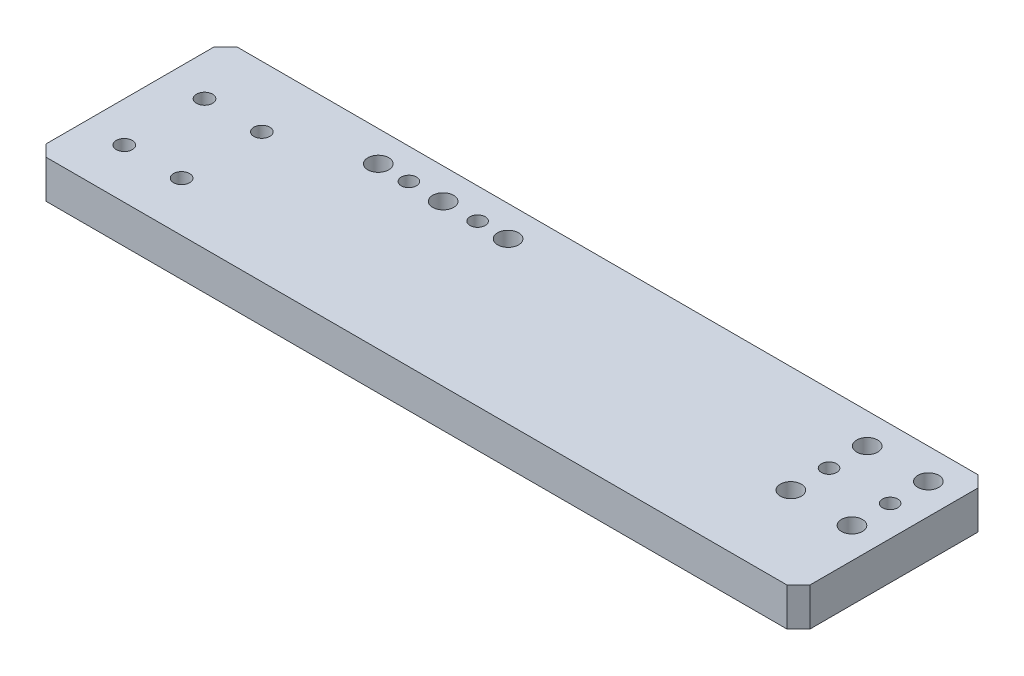
SolidWorks part; units mm, degrees
material "A6061 T6"
ref_plane "前视基准面" through (0, 0, 0) normal (0, 0, 1) x (1, 0, 0)
ref_plane "上视基准面" through (0, 0, 0) normal (0, 1, 0) x (1, 0, 0)
ref_plane "右视基准面" through (0, 0, 0) normal (1, 0, 0) x (0, 0, -1)
sketch "草图6" plane through (0, 0, 0) normal (0, 1, 0) x (1, 0, 0)
  line L1 (-100, 25) -> (100, 25)
  line L2 (-100, 25) -> (-100, -25)
  line L3 (-100, -25) -> (100, -25)
  line L4 (100, 25) -> (100, -25)
  line L5 (-100, 25) -> (100, -25) construction
  line L6 (-100, -25) -> (100, 25) construction
  point P0 (0, 0)
  dimension "D1" = 200
  dimension "D2" = 50
extrude "凸台-拉伸1" add sketch "草图6" along normal blind 10
chamfer "倒角1" distance 3 angle 45 4 edges at (100, 5, 25) (100, 5, -25) (-100, 5, 25) (-100, 5, -25)
hole_wizard "Ø5.5 (5.5) 直径孔1" positions "草图16" profile "草图17" hole size "Ø5.5" standard "GB"
sketch "草图16" plane through (0, 10, 0) normal (0, 1, 0) x (1, 0, 0)
  line L0 (-97, -25) -> (97, -25) construction
  line L1 (100, -22) -> (100, 22) construction
  point P0 (76, 17)
  point P2 (76, -3)
  point P4 (92, -3)
  point P6 (92, 17)
  dimension "D1" = 22
  dimension "D2" = 20
  dimension "D3" = 8
  dimension "D4" = 16
sketch "草图17" plane through (76, 10, -17) normal (1, 0, 0) x (0, 0, 1)
  line L0 (0, 0) -> (0, 14.0524)
  line L1 (0, 14.0524) -> (2.75, 12.4)
  line L2 (2.75, 12.4) -> (2.75, 0)
  line L5 (2.75, 0) -> (0, 0)
  line L10 (0, 14.0524) -> (-2.75, 12.4) construction
  line L11 (0, -6.35) -> (0, 107.95) construction
  dimension "孔直径" = 5.5
  dimension "孔深度" = 12.4
  dimension "导头角度" = 118
hole_wizard "大小mm 暗销孔2" positions "草图18" profile "草图19" hole size "Ø4.0" standard "GB"
sketch "草图18" plane through (0, 10, 0) normal (0, 1, 0) x (1, 0, 0)
  line L0 (100, -22) -> (100, 22) construction
  line L1 (-97, -25) -> (97, -25) construction
  point P0 (76, 7)
  point P2 (92, 7)
  dimension "D1" = 8
  dimension "D2" = 16
  dimension "D3" = 32
sketch "草图19" plane through (76, 10, -7) normal (1, 0, 0) x (0, 0, 1)
  line L0 (0, 0) -> (0, 13.6017)
  line L1 (0, 13.6017) -> (2, 12.4)
  line L2 (2, 12.4) -> (2, 0)
  line L5 (2, 0) -> (0, 0)
  line L10 (0, 13.6017) -> (-2, 12.4) construction
  line L11 (0, -6.35) -> (0, 107.95) construction
  dimension "孔直径" = 4
  dimension "孔深度" = 12.4
  dimension "导头角度" = 118
hole_wizard "M5 螺纹孔2" positions "草图20" profile "草图21" tap size "M5" standard "GB"
sketch "草图20" plane through (0, 10, 0) normal (0, 1, 0) x (1, 0, 0)
  point P0 (-89.5, 9)
  point P3 (-74.5, 9)
  point P6 (-89.5, -12)
  point P9 (-74.5, -12)
sketch "草图21" plane through (-89.5, 10, -9) normal (1, 0, 0) x (0, 0, 1)
  line L0 (0, 0) -> (0, 13.6618)
  line L1 (0, 13.6618) -> (2.1, 12.4)
  line L2 (2.1, 12.4) -> (2.1, 0)
  line L5 (2.1, 0) -> (0, 0)
  line L10 (0, 13.6618) -> (-2.1, 12.4) construction
  line L11 (0, -6.35) -> (0, 107.95) construction
  dimension "螺纹孔钻头直径" = 4.2
  dimension "螺纹孔钻头深度" = 12.4
  dimension "导头角度" = 118
cosmetic thread "孔螺蚊线4" parameters "D1"=10, "D2"=5
cosmetic thread "孔螺蚊线5" parameters "D1"=10, "D2"=5
cosmetic thread "孔螺蚊线6" parameters "D1"=10, "D2"=5
cosmetic thread "孔螺蚊线7" parameters "D1"=10, "D2"=5
hole_wizard "Ø5.5 (5.5) 直径孔2" positions "草图22" profile "草图24" hole size "Ø5.5" standard "GB"
sketch "草图22" plane through (0, 0, 0) normal (0, -1, 0) x (-1, 0, 0)
  point P0 (52, 17)
  point P3 (35, 16.9743)
  point P6 (18, 16.9743)
sketch "草图24" plane through (-52, 0, -17) normal (1, 0, 0) x (0, 0, -1)
  line L0 (0, 0) -> (0, 14.0524)
  line L1 (0, 14.0524) -> (2.75, 12.4)
  line L2 (2.75, 12.4) -> (2.75, 0)
  line L5 (2.75, 0) -> (0, 0)
  line L10 (0, 14.0524) -> (-2.75, 12.4) construction
  line L11 (0, -6.35) -> (0, 107.95) construction
  dimension "孔直径" = 5.5
  dimension "孔深度" = 12.4
  dimension "导头角度" = 118
hole_wizard "大小mm 暗销孔3" positions "草图25" profile "草图26" hole size "Ø4.0" standard "GB"
sketch "草图25" plane through (0, 0, 0) normal (0, -1, 0) x (-1, 0, 0)
  point P0 (44, 17)
  point P3 (26, 17)
sketch "草图26" plane through (-44, 0, -17) normal (1, 0, 0) x (0, 0, -1)
  line L0 (0, 0) -> (0, 13.6017)
  line L1 (0, 13.6017) -> (2, 12.4)
  line L2 (2, 12.4) -> (2, 0)
  line L5 (2, 0) -> (0, 0)
  line L10 (0, 13.6017) -> (-2, 12.4) construction
  line L11 (0, -6.35) -> (0, 107.95) construction
  dimension "孔直径" = 4
  dimension "孔深度" = 12.4
  dimension "导头角度" = 118
